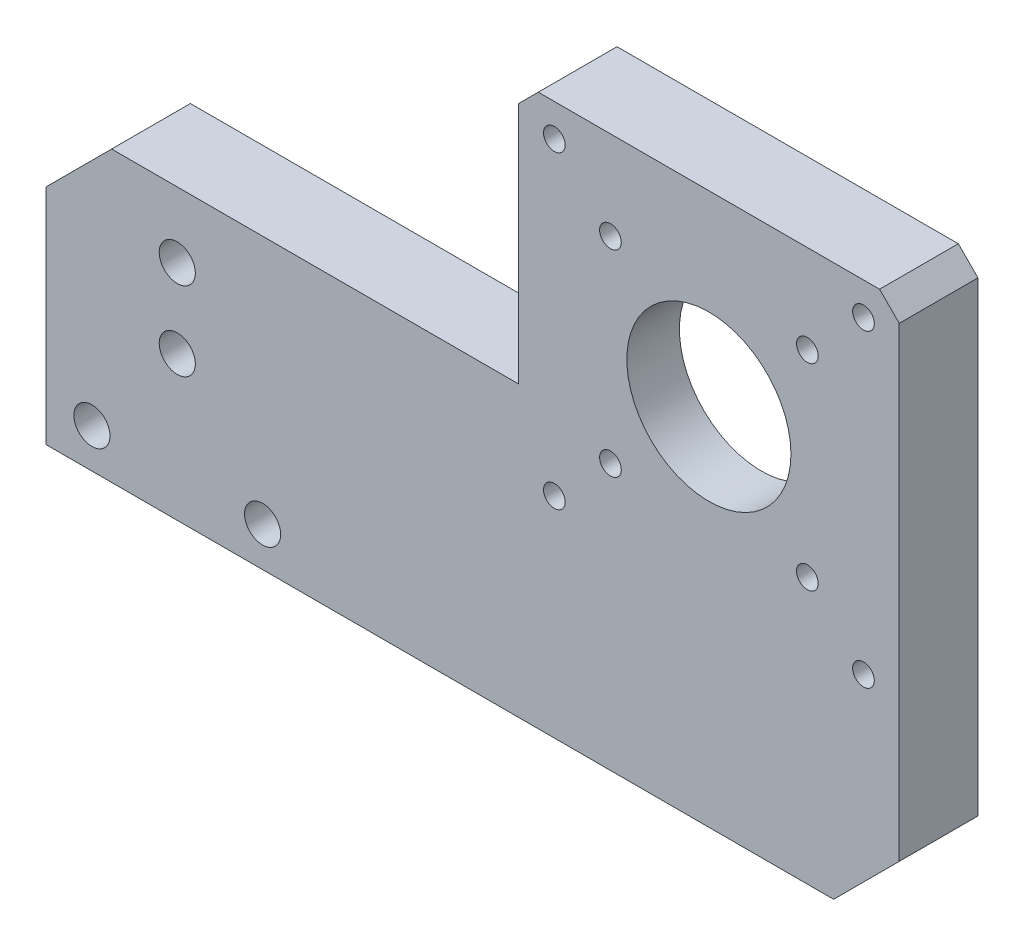
from build123d import *

# Parameters (mm, degrees)
SKETCH_1_W                  = 58
SKETCH_1_H                  = 103.5
EXTRUDE_1_DEPTH             = 12
HOLE_WIZARD_M4_1_D          = 3.3
SKETCH_5_R                  = 20
CUT_EXTRUDE_1_DEPTH         = 61.523239338
SKETCH_6_W                  = 58
SKETCH_6_H                  = 58
EXTRUDE_2_DEPTH             = 10
SKETCH_10_W                 = 48
SKETCH_10_H                 = 10
CUT_EXTRUDE_2_DEPTH         = 146
CHAMFER_1_SIZE              = 3
CUT_EXTRUDE_5_DEPTH         = 86.56320763
CUT_EXTRUDE_5_DEPTH_BACK    = 86.56320763
SKETCH_15_W                 = 130
SKETCH_15_H                 = 14
EXTRUDE_3_DEPTH             = 12
SKETCH_16_W                 = 40
SKETCH_16_H                 = 14
EXTRUDE_4_DEPTH             = 60
EXTRUDE_START               = -40
SKETCH_17_W                 = 12
SKETCH_17_H                 = 100
EXTRUDE_5_DEPTH             = 40
EXTRUDE_START_2             = -12
SKETCH_18_W                 = 72
SKETCH_18_H                 = 30
EXTRUDE_6_DEPTH             = 12
CHAMFER_2_SIZE              = 10
SKETCH_19_R                 = 22.248352005
SKETCH_19_R_2               = 12.5
EXTRUDE_7_DEPTH             = 8
CUT_EXTRUDE_6_DEPTH         = 158.012738337
CUT_EXTRUDE_6_DEPTH_BACK    = 158.012738337
HOLE_WIZARD_C_0_D           = 5.5
HOLE_WIZARD_C_0_CBORE_D     = 10
HOLE_WIZARD_C_0_CBORE_DEPTH = 5.5
CHAMFER_3_SIZE              = 10
HOLE_WIZARD_M4_2_D          = 3.3


with BuildPart() as part:
    # 草图1 → 凸台-拉伸1 (new body)
    with BuildSketch(Plane.XY):
        Rectangle(SKETCH_1_W, SKETCH_1_H)
    extrude(amount=EXTRUDE_1_DEPTH)

    # M4 螺纹孔1 (through all)
    with Locations(Plane(origin=(0, 0, 0), x_dir=(-1, 0, 0), z_dir=(0, 0, -1))):
        with Locations((-23.55, 46.8), (23.55, 46.8), (23.55, -0.3), (-23.55, -0.3)):
            Hole(HOLE_WIZARD_M4_1_D / 2)

    # 草图5 → 切除-拉伸1 (cut, through all)
    with BuildSketch(Plane(origin=(0, 0, 0), x_dir=(-1, 0, 0), z_dir=(0, 0, -1))):
        with Locations((0, 23.25)):
            Circle(SKETCH_5_R)
    extrude(amount=-CUT_EXTRUDE_1_DEPTH, mode=Mode.SUBTRACT)

    # 草图6 → 凸台-拉伸2 (add)
    with BuildSketch(Plane.XZ.offset(51.75)):
        with Locations((0, 29)):
            Rectangle(SKETCH_6_W, SKETCH_6_H)
    extrude(amount=EXTRUDE_2_DEPTH)

    # 草图10 → 切除-拉伸2 (cut)
    with BuildSketch(Plane(origin=(29, 0, 0), x_dir=(0, 0, -1), z_dir=(1, 0, 0))):
        with Locations((-36, -56.75)):
            Rectangle(SKETCH_10_W, SKETCH_10_H)
    extrude(amount=-CUT_EXTRUDE_2_DEPTH, mode=Mode.SUBTRACT)

    # 倒角1
    chamfer_1_edges = [part.edges().sort_by_distance(p)[0] for p in [
        (29, -61.75, 6),
        (-29, -61.75, 6),
        (-29, 51.75, 6),
        (29, 51.75, 6),
    ]]
    chamfer(chamfer_1_edges, length=CHAMFER_1_SIZE)

    # 草图14 → 切除-拉伸5 (cut, two sides: drawn at the far end of the back side and taken through both)
    with BuildSketch(Plane.ZY.offset(29).offset(-CUT_EXTRUDE_5_DEPTH_BACK)):
        Polygon((-205.249277876, -18.25), (-30, -18.25), (43.895682699, -18.25), (219.144960575, -18.25), (219.144960575, -368.748555752), (-205.249277876, -368.748555752), align=None)
    extrude(amount=CUT_EXTRUDE_5_DEPTH + CUT_EXTRUDE_5_DEPTH_BACK, mode=Mode.SUBTRACT)

    # 草图15 → 凸台-拉伸3 (add)
    with BuildSketch(Plane(origin=(0, 0, 0), x_dir=(-1, 0, 0), z_dir=(0, 0, -1))):
        with Locations((36, -25.25)):
            Rectangle(SKETCH_15_W, SKETCH_15_H)
    extrude(amount=-EXTRUDE_3_DEPTH)

    # 草图16 → 凸台-拉伸4 (add)
    with BuildSketch(Plane.XY.offset(12)):
        with Locations((-81, -25.25)):
            Rectangle(SKETCH_16_W, SKETCH_16_H)
    extrude(amount=EXTRUDE_4_DEPTH)

    # 草图17 → 凸台-拉伸5 (add)
    with BuildSketch(Plane.ZY.offset(101).offset(EXTRUDE_START)):
        with Locations((78, -68.25)):
            Rectangle(SKETCH_17_W, SKETCH_17_H)
    extrude(amount=EXTRUDE_5_DEPTH)

    # 草图18 → 凸台-拉伸6 (add)
    with BuildSketch(Plane(origin=(0, 0, 0), x_dir=(-1, 0, 0), z_dir=(0, 0, -1)).offset(EXTRUDE_START_2)):
        with Locations((65, -3.25)):
            Rectangle(SKETCH_18_W, SKETCH_18_H)
    extrude(amount=EXTRUDE_6_DEPTH)

    # 倒角2
    chamfer_2_edges = [part.edges().sort_by_distance(p)[0] for p in [
        (29, -32.25, 6),
    ]]
    chamfer(chamfer_2_edges, length=CHAMFER_2_SIZE)

    # 草图19 → 凸台-拉伸7 (add)
    with BuildSketch(Plane.XY.offset(12)):
        with Locations((0, 23.25)):
            Circle(SKETCH_19_R)
        with Locations((0, 23.25)):
            Circle(SKETCH_19_R_2, mode=Mode.SUBTRACT)
    extrude(amount=-EXTRUDE_7_DEPTH)

    # 草图20 → 切除-拉伸6 (cut, two sides: drawn at the far end of the back side and taken through both)
    with BuildSketch(Plane.XZ.offset(32.25).offset(-CUT_EXTRUDE_6_DEPTH_BACK)):
        Polygon((259.644501793, 12), (-52.844544679, 12), (-104.007164502, 12), (-416.496210973, 12), (-416.496210973, 636.978092943), (259.644501793, 636.978092943), align=None)
    extrude(amount=CUT_EXTRUDE_6_DEPTH + CUT_EXTRUDE_6_DEPTH_BACK, mode=Mode.SUBTRACT)

    # 打孔尺寸根据六角头螺栓 C 级的类型0 (through all)
    with Locations(Plane(origin=(0, 0, 0), x_dir=(-1, 0, 0), z_dir=(0, 0, -1))):
        with Locations((72.148493823, 215.242463417), (94, -26.25), (68, -26.25), (81, -10.25), (81, 1.75)):
            CounterBoreHole(HOLE_WIZARD_C_0_D / 2, HOLE_WIZARD_C_0_CBORE_D / 2, HOLE_WIZARD_C_0_CBORE_DEPTH)

    # 倒角3
    chamfer_3_edges = [part.edges().sort_by_distance(p)[0] for p in [
        (-101, 11.75, 6),
    ]]
    chamfer(chamfer_3_edges, length=CHAMFER_3_SIZE)

    # M4 螺纹孔2 (through all)
    with Locations(Plane.XY.offset(12)):
        with Locations((15, 8.25), (-15, 8.25), (-15, 38.25), (15, 38.25)):
            Hole(HOLE_WIZARD_M4_2_D / 2)


solid = part.part
